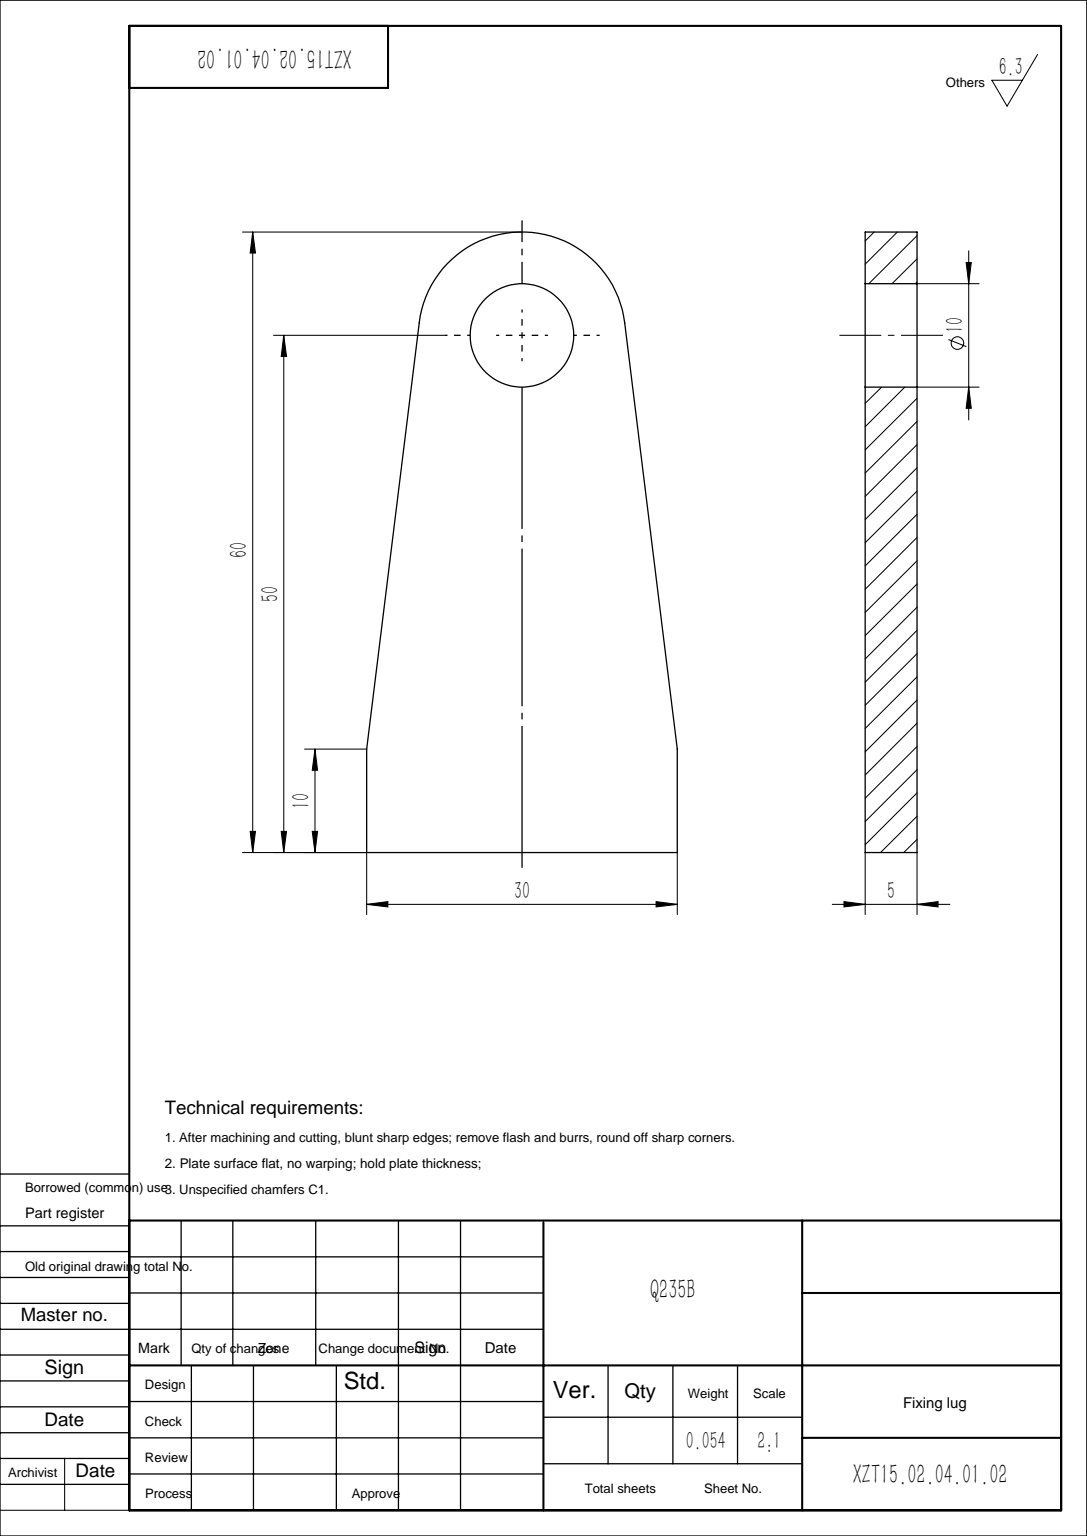
from build123d import *

# Parameters (mm, degrees)
SKETCH1_R           = 5
BOSS_EXTRUDE1_DEPTH = 2.5
SKETCH2_W           = 30
SKETCH2_H           = 10
BOSS_EXTRUDE2_DEPTH = 5


with BuildPart() as part:
    # Sketch1 → Boss-Extrude1 (new, symmetric)
    with BuildSketch(Plane.XY):
        with BuildLine():
            Line((15, 0), (-15, 0))
            Line((-15, 0), (-9.925067247, 41.221900218))
            ThreePointArc((-9.925067247, 41.221900218), (0, 50), (9.925067247, 41.221900218))
            Line((9.925067247, 41.221900218), (15, 0))
        make_face()
        with Locations((0, 40)):
            Circle(SKETCH1_R, mode=Mode.SUBTRACT)
    extrude(amount=BOSS_EXTRUDE1_DEPTH, both=True)

    # Sketch2 → Boss-Extrude2 (add)
    with BuildSketch(Plane.XY.offset(2.5)):
        with Locations((0, -5)):
            Rectangle(SKETCH2_W, SKETCH2_H)
    extrude(amount=-BOSS_EXTRUDE2_DEPTH)


solid = part.part
